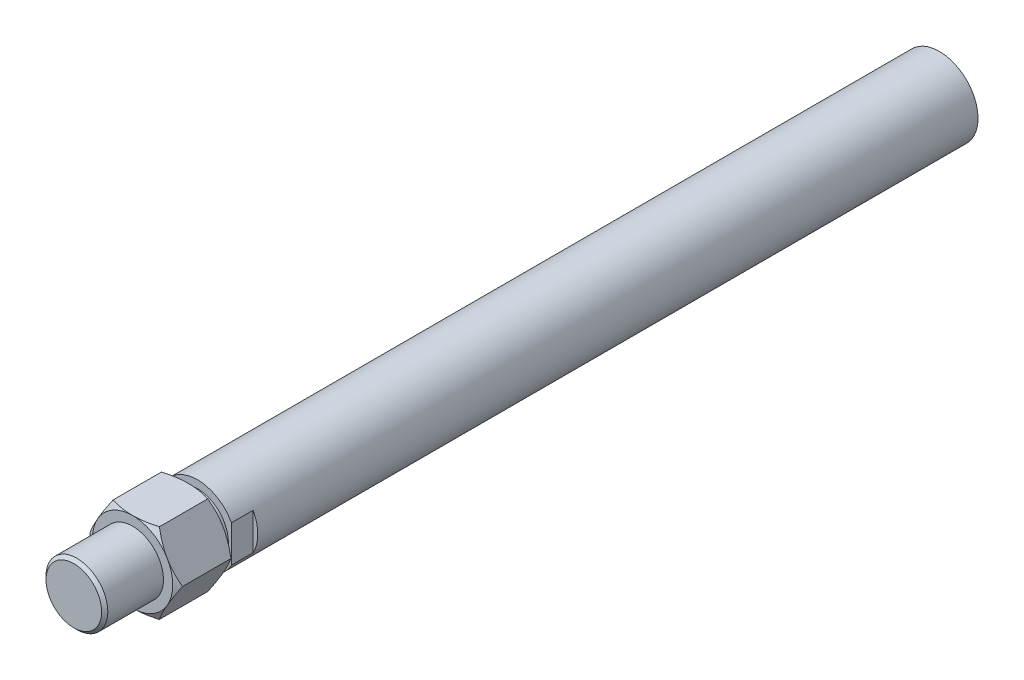
from build123d import *

# Parameters (mm, degrees)
SKETCH5_OUTSIDE_W  = 88.64
SKETCH5_OUTSIDE_H  = 88.64
CUT_EXTRUDE1_DEPTH = 18
SKETCH6_OUTSIDE_W  = 123.2
SKETCH6_OUTSIDE_H  = 119.18
SKETCH6_OUTSIDE_R  = 12.990381057
CUT_EXTRUDE2_DEPTH = 10
CUT_EXTRUDE2_DRAFT = -60
SKETCH7_OUTSIDE_W  = 123.2
SKETCH7_OUTSIDE_H  = 119.18
SKETCH7_OUTSIDE_R  = 12.990381057
CUT_EXTRUDE3_DEPTH = 10
CUT_EXTRUDE3_DRAFT = -60
SKETCH9_W          = 22
SKETCH9_H          = 25.980762114
CUT_EXTRUDE4_DEPTH = 7
CHAMFER1_SIZE      = 1


with BuildPart() as part:
    # Sketch3 → Revolve1 (revolve)
    with BuildSketch(Plane(origin=(0, 0, 0), x_dir=(0, 0, -1), z_dir=(1, 0, 0)), mode=Mode.PRIVATE) as revolve1_sk:
        Polygon((-38, 12.5), (-38, 0), (-318, 0), (-318, 10), (-299, 10), (-299, 15), (-281, 15), (-281, 10), (-278, 10), (-278, 12.5), align=None)
    revolve(revolve1_sk.sketch.rotate(Axis((0, 0, 318), (0, 0, -1)), 180), axis=Axis((0, 0, 318), (0, 0, -1)))

    # Sketch5 outside → Cut-Extrude1 (cut)
    with BuildSketch(Plane.XY.offset(299)):
        Rectangle(SKETCH5_OUTSIDE_W, SKETCH5_OUTSIDE_H)
        Polygon((7.5, 12.990381057), (-7.5, 12.990381057), (-15, 0), (-7.5, -12.990381057), (7.5, -12.990381057), (15, 0), align=None, mode=Mode.SUBTRACT)
    extrude(amount=-CUT_EXTRUDE1_DEPTH, mode=Mode.SUBTRACT)


with BuildPart() as cut_extrude2_tool:
    # Sketch6 outside → Cut-Extrude2 (with draft: the straight prism first)
    with BuildSketch(Plane.XY.offset(299)):
        Rectangle(SKETCH6_OUTSIDE_W, SKETCH6_OUTSIDE_H)
        Circle(SKETCH6_OUTSIDE_R, mode=Mode.SUBTRACT)
    extrude(amount=-CUT_EXTRUDE2_DEPTH)
    # Cut-Extrude2: the draft: its side faces are tilted about the plane it starts from
    cut_extrude2_sides = [cut_extrude2_tool.faces().sort_by_distance(p)[0] for p in [
        (0, -59.59, 294),
        (61.6, 0, 294),
        (0, 59.59, 294),
        (-61.6, 0, 294),
        (-12.990381057, 0, 294),
    ]]
    draft(cut_extrude2_sides, Plane.XY.offset(299), CUT_EXTRUDE2_DRAFT)


with BuildPart() as part_1:
    add(part.part)

    # Cut-Extrude2: cut by cut_extrude2_tool
    add(cut_extrude2_tool.part, mode=Mode.SUBTRACT)


with BuildPart() as cut_extrude3_tool:
    # Sketch7 outside → Cut-Extrude3 (with draft: the straight prism first)
    with BuildSketch(Plane(origin=(0, 0, 281), x_dir=(-1, 0, 0), z_dir=(0, 0, -1))):
        Rectangle(SKETCH7_OUTSIDE_W, SKETCH7_OUTSIDE_H)
        Circle(SKETCH7_OUTSIDE_R, mode=Mode.SUBTRACT)
    extrude(amount=-CUT_EXTRUDE3_DEPTH)
    # Cut-Extrude3: the draft: its side faces are tilted about the plane it starts from
    cut_extrude3_sides = [cut_extrude3_tool.faces().sort_by_distance(p)[0] for p in [
        (0, -59.59, 286),
        (-61.6, 0, 286),
        (0, 59.59, 286),
        (61.6, 0, 286),
        (12.990381057, 0, 286),
    ]]
    draft(cut_extrude3_sides, Plane(origin=(0, 0, 281), x_dir=(-1, 0, 0), z_dir=(0, 0, -1)), CUT_EXTRUDE3_DRAFT)


with BuildPart() as part_2:
    add(part_1.part)

    # Cut-Extrude3: cut by cut_extrude3_tool
    add(cut_extrude3_tool.part, mode=Mode.SUBTRACT)

    # Sketch9 → Cut-Extrude4 (cut)
    with BuildSketch(Plane.XY.offset(278)):
        with Locations((-22, 0)):
            Rectangle(SKETCH9_W, SKETCH9_H)
        with Locations((22, 0)):
            Rectangle(SKETCH9_W, SKETCH9_H)
    extrude(amount=-CUT_EXTRUDE4_DEPTH, mode=Mode.SUBTRACT)

    # Chamfer1
    chamfer1_edges = [part_2.edges().sort_by_distance(p)[0] for p in [
        (0, 10, 318),
    ]]
    chamfer(chamfer1_edges, length=CHAMFER1_SIZE)


solid = part_2.part
